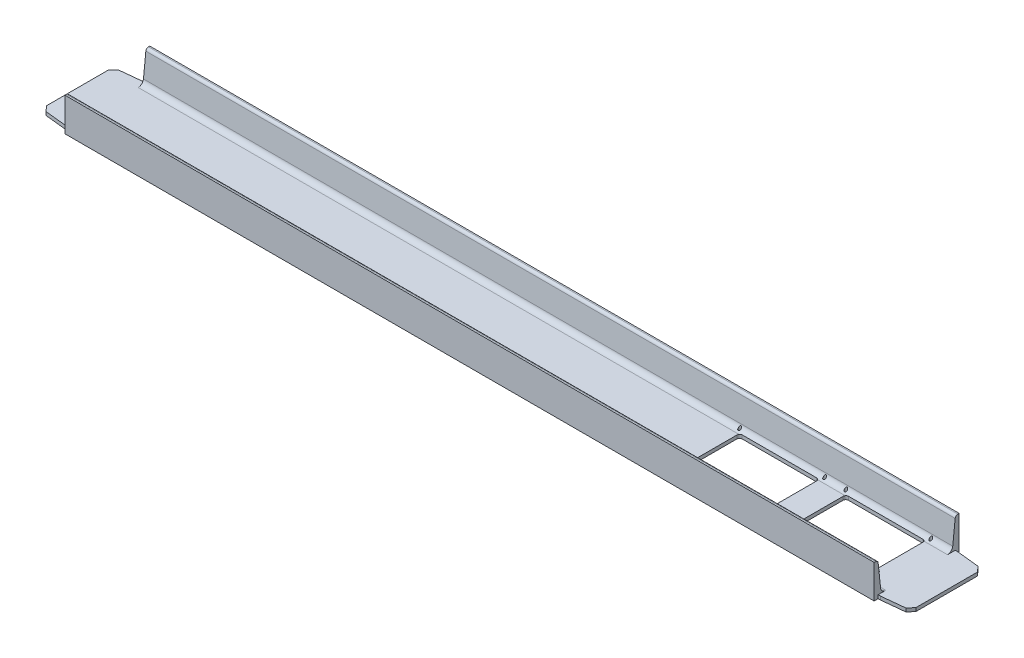
SolidWorks part; units mm, degrees
material "Q235B"
ref_plane "前视基准面" through (0, 0, 0) normal (0, 0, 1) x (1, 0, 0)
ref_plane "上视基准面" through (0, 0, 0) normal (0, 1, 0) x (1, 0, 0)
ref_plane "右视基准面" through (0, 0, 0) normal (1, 0, 0) x (0, 0, -1)
other "Configuration Table"
sketch "草图1" plane through (0, 0, 0) normal (0, 0, 1) x (1, 0, 0)
  line L0 (-818.5, 0) -> (818.5, 0)
  point P3 (0, 0)
  dimension "D1" = 1637
other "Gbt706-2008 热轧槽钢 16A(1)"
ref_plane "基准面1" through (-818.5, 0, 0) normal (1, 0, 0) x (0, 1, 0)
sketch "Sketch12" plane through (-818.5, 0, 0) normal (1, 0, 0) x (0, 1, 0)
  line L0 (63, 160) -> (0, 160)
  line L1 (63, 0) -> (0, 0)
  line L2 (0, 160) -> (0, 0)
  line L3 (-9.5694, 80) -> (49.7414, 80) construction
  line L4 (6.5, 138.0268) -> (6.5, 21.9732)
  line L5 (63, 0) -> (63, 2.5288)
  line L6 (63, 160) -> (63, 157.4712)
  line L7 (15.4547, 12.028) -> (58.5226, 7.5014)
  line L17 (15.4547, 147.972) -> (58.5226, 152.4986)
  arc A0 (58.5226, 152.4986) -> (63, 157.4712) centre (58, 157.4712) ccw
  arc A1 (58.5226, 7.5014) -> (63, 2.5288) centre (58, 2.5288) cw
  arc A2 (6.5, 21.9732) -> (15.4547, 12.028) centre (16.5, 21.9732) ccw
  arc A10 (6.5, 138.0268) -> (15.4547, 147.972) centre (16.5, 138.0268) cw
  point P6 (0, 0)
  point P8 (0, 80)
  point P9 (6.5, 25.8841)
  point P10 (31.5, 160)
  point P13 (63, 152.9692)
  point P14 (34.75, 150)
  point P19 (6.5, 80)
sketch "草图2" plane through (0, 0, 0) normal (0, -1, 0) x (1, 0, 0)
  line L0 (762, -5) -> (762, 7.5014)
  line L3 (-766.4774, 7.5014) -> (766.4774, 7.5014) construction
  line L4 (762, 7.5014) -> (766.4774, 7.5014)
  line L5 (766.4774, 7.5014) -> (809.5453, 12.028)
  line L6 (809.5453, 12.028) -> (818.5, 21.9732)
  line L7 (818.5, 21.9732) -> (818.5, 138.0268)
  line L8 (818.5, 138.0268) -> (809.5453, 147.972)
  line L9 (809.5453, 147.972) -> (766.4774, 152.4986)
  line L10 (766.4774, 152.4986) -> (762, 152.4986)
  line L11 (-766.4774, 152.4986) -> (766.4774, 152.4986) construction
  line L12 (762, 152.4986) -> (762, 165)
  line L14 (762, 165) -> (828.5, 165)
  line L15 (828.5, 165) -> (828.5, -5)
  line L16 (828.5, -5) -> (762, -5)
  line L18 (818.5, 0) -> (-818.5, 0) construction
  line L19 (818.5, 160) -> (-818.5, 160) construction
  line L20 (818.5, 160) -> (818.5, 0) construction
  dimension "D1" = 5
  dimension "D2" = 5
  dimension "D3" = 10
  dimension "D4" = 56.5
extrude "切除-拉伸1" cut sketch "草图2" against normal through all
sketch "草图3" plane through (0, 0, 0) normal (0, -1, 0) x (1, 0, 0)
  line L0 (-762, 0) -> (-762, 7.5014)
  line L1 (762, 0) -> (-818.5, 0) construction
  line L2 (-762, 2.5288) -> (-762, 0) construction
  line L3 (-766.4774, 7.5014) -> (766.4774, 7.5014) construction
  line L4 (-762, 7.5014) -> (-766.4774, 7.5014)
  line L5 (-766.4774, 7.5014) -> (-809.5453, 12.028)
  line L6 (-809.5453, 12.028) -> (-818.5, 21.9732)
  line L7 (-818.5, 160) -> (-818.5, 0) construction
  line L8 (-818.5, 21.9732) -> (818.5, 21.9732) construction
  line L9 (-818.5, 21.9732) -> (-818.5, 138.0268)
  line L10 (-818.5, 138.0268) -> (-809.5453, 147.972)
  line L11 (-809.5453, 147.972) -> (-766.4774, 152.4986)
  line L12 (-766.4774, 152.4986) -> (-762, 152.4986)
  line L13 (-766.4774, 152.4986) -> (766.4774, 152.4986) construction
  line L14 (-762, 152.4986) -> (-762, 165)
  line L15 (-762, 165) -> (-838.5, 165)
  line L16 (-838.5, 165) -> (-838.5, -5)
  line L17 (-838.5, -5) -> (-762, -5)
  line L18 (-762, -5) -> (-762, 0)
  line L19 (762, 160) -> (-818.5, 160) construction
  dimension "D1" = 20
  dimension "D2" = 5
  dimension "D3" = 5
extrude "切除-拉伸2" cut sketch "草图3" against normal through all
sketch "草图4" plane through (0, 0, 152.4986) normal (0, 0, 1) x (1, 0, 0)
  line L0 (818.5, 0) -> (818.5, 6.5) construction
  line L1 (818.5, 6.5) -> (762, 6.5)
  line L2 (818.5, 6.5) -> (818.5, 63)
  line L3 (818.5, 63) -> (762, 63)
  line L4 (762, 6.5) -> (762, 63)
  ellipse E0 centre (818.5, 16.5) end of major axis (818.5, 6.5) minor radius 9.004 (809.5453, 15.4547) -> (818.5, 6.5) ccw construction
extrude "切除-拉伸3" cut sketch "草图4" against normal through all
sketch "草图5" plane through (0, 0, 152.4986) normal (0, 0, 1) x (1, 0, 0)
  line L1 (-818.5, 6.5) -> (-762, 6.5)
  line L2 (-818.5, 6.5) -> (-818.5, 63)
  line L3 (-818.5, 63) -> (-762, 63)
  line L4 (-762, 6.5) -> (-762, 63)
extrude "切除-拉伸4" cut sketch "草图5" against normal through all
sketch "草图6" plane through (0, 0, 0) normal (0, -1, 0) x (1, 0, 0)
  line L0 (-772.2929, 0) -> (-107.7071, 0) construction
  line L1 (513.5, 20) -> (373.5, 20)
  line L2 (518.5, 25) -> (518.5, 105)
  line L3 (513.5, 110) -> (373.5, 110)
  line L4 (368.5, 25) -> (368.5, 105)
  line L5 (762, 160) -> (-762, 160) construction
  line L7 (718.5, 25) -> (718.5, 105)
  line L8 (713.5, 20) -> (573.5, 20)
  line L9 (568.5, 25) -> (568.5, 105)
  line L10 (713.5, 110) -> (573.5, 110)
  line L11 (518.5, 25) -> (718.5, 25) construction
  line L12 (818.5, 138.0268) -> (818.5, 21.9732) construction
  arc A0 (373.5, 110) -> (368.5, 105) centre (373.5, 105) ccw
  arc A1 (513.5, 110) -> (518.5, 105) centre (513.5, 105) cw
  arc A2 (368.5, 25) -> (373.5, 20) centre (373.5, 25) ccw
  arc A3 (513.5, 20) -> (518.5, 25) centre (513.5, 25) ccw
  arc A4 (713.5, 20) -> (718.5, 25) centre (713.5, 25) ccw
  arc A5 (568.5, 25) -> (573.5, 20) centre (573.5, 25) ccw
  arc A6 (573.5, 110) -> (568.5, 105) centre (573.5, 105) ccw
  arc A7 (713.5, 110) -> (718.5, 105) centre (713.5, 105) cw
  point P16 (368.5, 20)
  point P19 (518.5, 20)
  dimension "D5" = 5
  dimension "D1" = 20
  dimension "D2" = 50
  dimension "D3" = 100
  dimension "D4" = 150
  dimension "D7" = 200
  dimension "D6" = 2
extrude "切除-拉伸5" cut sketch "草图6" against normal up to next
hole_wizard "M6 螺纹孔1" positions "草图7" profile "草图8" tap size "M6" standard "GB" end condition through all
sketch "草图7" plane through (0, 0, 0) normal (0, -1, 0) x (-1, 0, 0)
  line L0 (-718.5, -25) -> (-718.5, -105) construction
  line L1 (-573.5, -20) -> (-713.5, -20) construction
  line L2 (-373.5, -20) -> (-513.5, -20) construction
  line L3 (-518.5, -25) -> (-518.5, -105) construction
  line L4 (-523.5, -15) -> (-363.5, -15) construction
  line L5 (-523.5, -15) -> (-523.5, -115) construction
  point P0 (-723.5, -15)
  point P9 (-523.5, -15)
  point P22 (-563.5, -15)
  point P23 (-363.5, -15)
  point P24 (-563.5, -115)
  point P25 (-363.5, -115)
  point P26 (-723.5, -115)
  point P27 (-523.5, -115)
  dimension "D1" = 5
  dimension "D2" = 5
  dimension "D3" = 5
  dimension "D4" = 5
  dimension "D7" = 160
  dimension "D8" = 100
  dimension "D5" = 2
  dimension "D6" = 2
sketch "草图8" plane through (723.5, 0, 15) normal (1, 0, 0) x (0, 0, -1)
  line L0 (0, 0) -> (0, 63)
  line L1 (0, 63) -> (2.5, 63)
  line L2 (2.5, 63) -> (2.5, 0)
  line L5 (2.5, 0) -> (0, 0)
  line L11 (0, -6.35) -> (0, 107.95) construction
  dimension "通孔螺纹孔钻头直径" = 5
  dimension "通孔螺纹孔钻头深度" = 63
cosmetic thread "孔螺蚊线1" parameters "D2"=6
cosmetic thread "孔螺蚊线2" parameters "D2"=6
cosmetic thread "孔螺蚊线3" parameters "D2"=6
cosmetic thread "孔螺蚊线4" parameters "D2"=6
cosmetic thread "孔螺蚊线5" parameters "D2"=6
cosmetic thread "孔螺蚊线6" parameters "D2"=6
cosmetic thread "孔螺蚊线7" parameters "D2"=6
cosmetic thread "孔螺蚊线8" parameters "D2"=6
equation "\"RI@Sketch12\"= \"D1@Sketch12\""
equation "\"D3@Sketch12\"=  ( \"BF@Sketch12\" - \"D6@Sketch12\" )  / 2"
